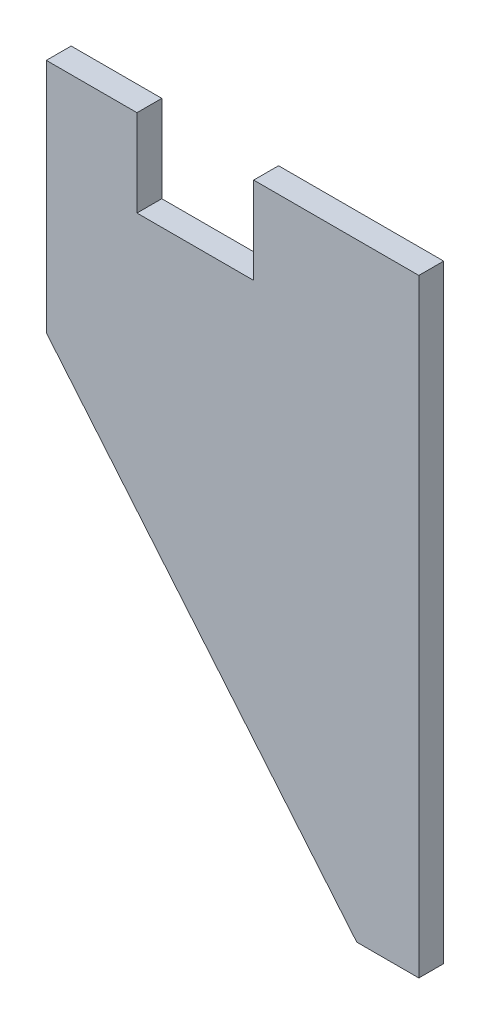
SolidWorks part; units mm, degrees
material "Q235"
ref_plane "Front Plane" through (0, 0, 0) normal (0, 0, 1) x (1, 0, 0)
ref_plane "Top Plane" through (0, 0, 0) normal (0, 1, 0) x (1, 0, 0)
ref_plane "Right Plane" through (0, 0, 0) normal (1, 0, 0) x (0, 0, -1)
sketch "Sketch1" plane through (0, 0, 0) normal (0, 0, 1) x (1, 0, 0)
  line L0 (0, 0) -> (0, -490)
  line L1 (0, -490) -> (-50, -490)
  line L2 (-50, -490) -> (-300, -190)
  line L3 (-300, -190) -> (-300, 0)
  line L4 (-300, 0) -> (-227, 0)
  line L5 (-227, 0) -> (-227, -70)
  line L6 (-227, -70) -> (-133, -70)
  line L7 (-133, -70) -> (-133, 0)
  line L8 (-133, 0) -> (0, 0)
  dimension "D1" = 133
  dimension "D2" = 94
  dimension "D3" = 490
  dimension "D4" = 70
  dimension "D5" = 300
  dimension "D6" = 190
  dimension "D7" = 50
extrude "Boss-Extrude1" add sketch "Sketch1" along normal blind 20
